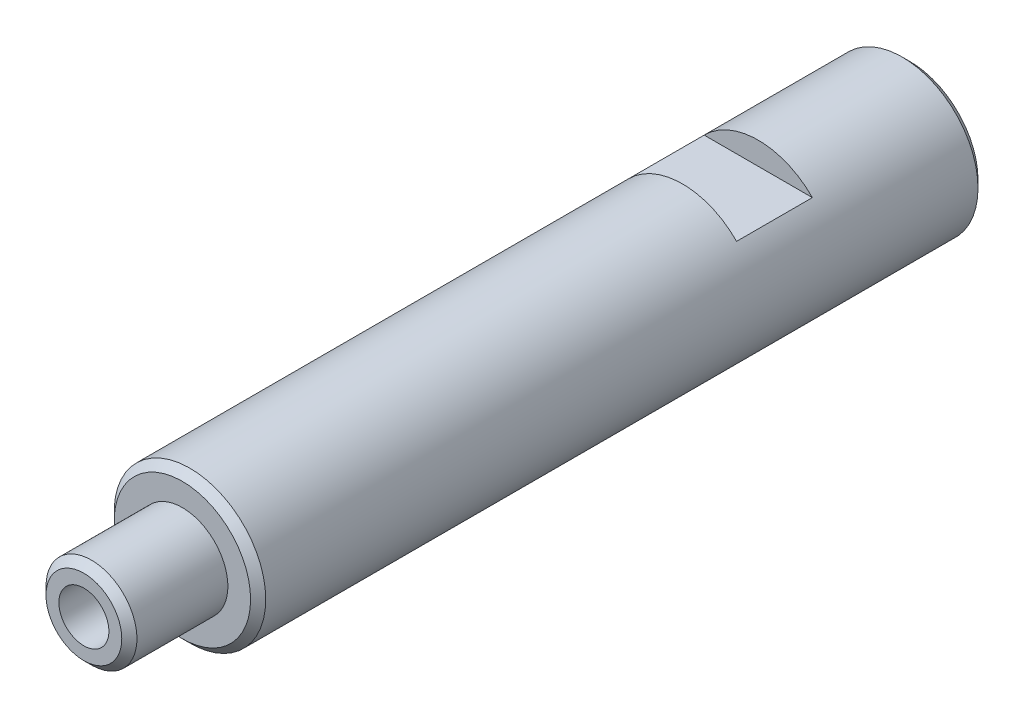
SolidWorks part; units mm, degrees
material "S45C"
ref_plane "Front Plane" through (0, 0, 0) normal (0, 0, 1) x (1, 0, 0)
ref_plane "Top Plane" through (0, 0, 0) normal (0, 1, 0) x (1, 0, 0)
ref_plane "Right Plane" through (0, 0, 0) normal (1, 0, 0) x (0, 0, -1)
sketch "Sketch1" plane through (0, 0, 0) normal (0, 0, 1) x (1, 0, 0)
  circle A0 centre (0, 0) radius 5
  dimension "D1" = 10
extrude "Boss-Extrude1" add sketch "Sketch1" along normal blind 48
sketch "Sketch2" plane through (0, 0, 48) normal (0, 0, 1) x (1, 0, 0)
  circle A0 centre (0, 0) radius 3
  dimension "D1" = 6
extrude "Boss-Extrude2" add sketch "Sketch2" along normal blind 6.5
hole_wizard "M4 Tapped Hole1" positions "Sketch4" profile "Sketch3" tap size "M4" standard "GB"
sketch "Sketch4" plane through (0, 0, 54.5) normal (0, 0, 1) x (1, 0, 0)
  point P0 (0, 0)
sketch "Sketch3" plane through (0, 0, 54.5) normal (1, 0, 0) x (0, -1, 0)
  line L0 (0, 0) -> (0, 11.0914)
  line L1 (0, 11.0914) -> (1.65, 10.1)
  line L2 (1.65, 10.1) -> (1.65, 0)
  line L5 (1.65, 0) -> (0, 0)
  line L10 (0, 11.0914) -> (-1.65, 10.1) construction
  line L11 (0, -6.35) -> (0, 107.95) construction
  dimension "螺纹孔钻头直径" = 3.3
  dimension "螺纹孔钻头深度" = 10.1
  dimension "导头角度" = 118
cosmetic thread "Cosmetic Thread1" parameters "D1"=8, "D2"=4
hole_wizard "M5 Tapped Hole1" positions "Sketch6" profile "Sketch5" tap size "M5" standard "GB"
sketch "Sketch6" plane through (0, 0, 0) normal (0, 0, -1) x (-1, 0, 0)
  point P0 (0, 0)
sketch "Sketch5" plane through (0, 0, 0) normal (1, 0, 0) x (0, 1, 0)
  line L0 (0, 0) -> (0, 13.6618)
  line L1 (0, 13.6618) -> (2.1, 12.4)
  line L2 (2.1, 12.4) -> (2.1, 0)
  line L5 (2.1, 0) -> (0, 0)
  line L10 (0, 13.6618) -> (-2.1, 12.4) construction
  line L11 (0, -6.35) -> (0, 107.95) construction
  dimension "螺纹孔钻头直径" = 4.2
  dimension "螺纹孔钻头深度" = 12.4
  dimension "导头角度" = 118
cosmetic thread "Cosmetic Thread2" parameters "D1"=10, "D2"=5
chamfer "Chamfer1" distance 0.5 angle 45 3 edges at (5, 0, 48) (5, 0, 0) (3, 0, 54.5)
sketch "Sketch7" plane through (0, 0, 0) normal (0, 1, 0) x (1, 0, 0)
  line L0 (-5, -0.5) -> (-5, -47.5) construction
  line L1 (-5, -10) -> (5, -10)
  line L2 (-5, -10) -> (-5, -15)
  line L3 (-5, -15) -> (5, -15)
  line L4 (5, -10) -> (5, -15)
  line L5 (5, -47.5) -> (5, -0.5) construction
  line L6 (4.5, 0) -> (-4.5, 0) construction
  dimension "D1" = 5
  dimension "D2" = 10
extrude "Cut-Extrude1" cut sketch "Sketch7" against normal mid plane 3 from offset 5
mirror "Mirror1" about plane through (0, 0, 0) normal (0, 1, 0) of "Cut-Extrude1"
